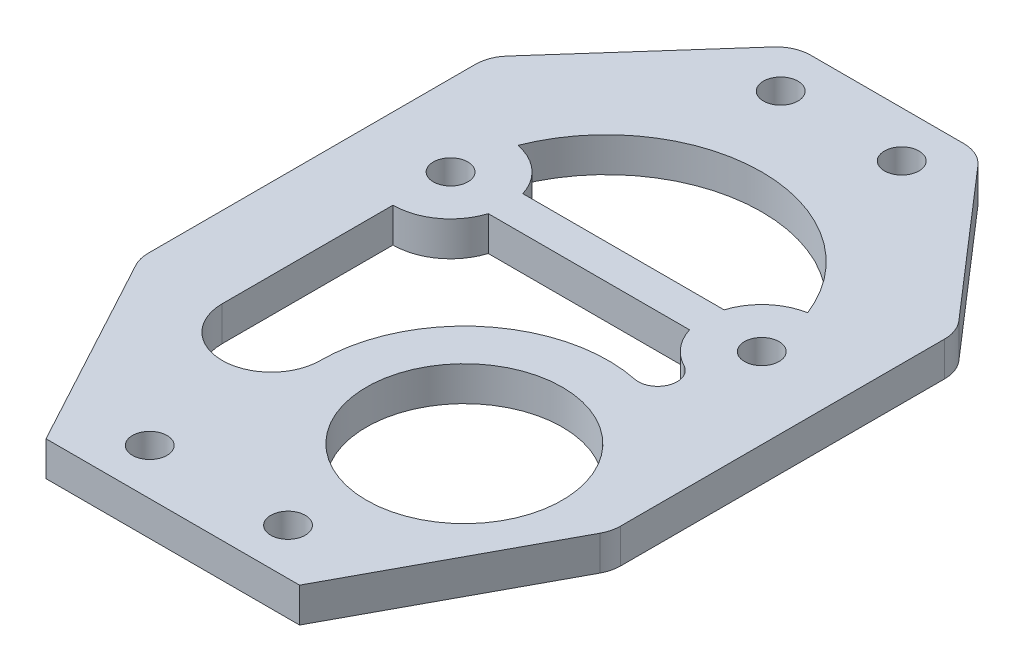
SolidWorks part; units mm, degrees
ref_plane "Front Plane" through (0, 0, 0) normal (0, 0, 1) x (1, 0, 0)
ref_plane "Top Plane" through (0, 0, 0) normal (0, 1, 0) x (1, 0, 0)
ref_plane "Right Plane" through (0, 0, 0) normal (1, 0, 0) x (0, 0, -1)
sketch "Sketch1" plane through (0, 0, 0) normal (0, 1, 0) x (1, 0, 0)
  line L0 (-11, 0) -> (11, 0)
  line L1 (0, 0) -> (0, 62) construction
  line L2 (-8, 62) -> (8, 62)
  line L3 (11, 0) -> (20.4896, 17.6053)
  line L4 (20.4896, 17.6053) -> (20.4896, 47.6053)
  line L5 (20.4896, 47.6053) -> (8, 62)
  line L6 (-11, 0) -> (-20.5092, 17.6107)
  line L7 (-20.5092, 17.6107) -> (-20.5092, 47.9103)
  line L8 (-20.5092, 47.9103) -> (-8, 62)
  line L9 (20.4896, 17.6053) -> (10.3666, 23.0618) construction
  line L10 (-5.25, 57.9999) -> (5.25, 57.9999) construction
  line L11 (-13.5, 37.6053) -> (13.5, 37.6053) construction
  line L12 (-8.7303, 39.1053) -> (8.7303, 39.1053)
  line L13 (-8.7303, 36.1053) -> (8.7303, 36.1053)
  line L14 (-13.5, 32.6053) -> (-13.5, 17.7879)
  circle A0 centre (7.5197, 17.7803) radius 8.5
  circle A1 centre (6, 4) radius 1.5
  circle A2 centre (-6, 4) radius 1.5
  circle A3 centre (-5.25, 57.9999) radius 1.5
  circle A4 centre (5.25, 57.9999) radius 1.5
  circle A5 centre (-13.5, 37.6053) radius 1.5
  circle A6 centre (13.5, 37.6053) radius 1.5
  arc A7 (-8.7303, 39.1053) -> (-12.5741, 42.5188) centre (-13.5, 37.6053) ccw
  arc A8 (10.0627, 30.0188) -> (-4.9803, 17.786) centre (7.5197, 17.7803) ccw
  arc A9 (8.7303, 36.1053) -> (11.188, 33.172) centre (13.5, 37.6053) ccw
  arc A10 (12.5741, 42.5188) -> (-12.5741, 42.5188) centre (0, 37.6053) ccw
  arc A11 (-13.5, 32.6053) -> (-8.7303, 36.1053) centre (-13.5, 37.6053) ccw
  arc A12 (-13.5, 17.7879) -> (-4.9803, 17.786) centre (-9.2402, 17.7879) ccw
  arc A13 (10.0627, 30.0188) -> (11.188, 33.172) centre (10.4065, 31.6735) ccw
  arc A14 (12.5741, 42.5188) -> (8.7303, 39.1053) centre (13.5, 37.6053) ccw
  point P7 (0, 62)
  point P17 (20.4896, 17.6053)
  point P24 (0, 57.9999)
  point P27 (0, 37.6053)
  dimension "D7" = 17
  dimension "D13" = 3
  dimension "D14" = 3
  dimension "D19" = 3
  dimension "D20" = 10
  dimension "D21" = 4
  dimension "D23" = 1.69
  dimension "D22" = 45
  dimension "D24" = 13.5
  dimension "D25" = 5
  dimension "D26" = 14.8174
  dimension "D27" = 3
  dimension "D1" = 22
  dimension "D2" = 16
  dimension "D3" = 62
  dimension "D4" = 20
  dimension "D5" = 30
  dimension "D6" = 41
  dimension "D8" = 11.5
  dimension "D9" = 11.5
  dimension "D10" = 6
  dimension "D11" = 4
  dimension "D12" = 12
  dimension "D15" = 10.5
  dimension "D16" = 22
  dimension "D17" = 10
  dimension "D18" = 27
extrude "Boss-Extrude1" add sketch "Sketch1" along normal blind 3
fillet "Fillet1" radius 3 6 edges at (8, 1.5, -62) (20.4896, 1.5, -47.6053) (20.4896, 1.5, -17.6053) (-20.5092, 1.5, -17.6107) (-8, 1.5, -62) (-20.5092, 1.5, -47.9103)
